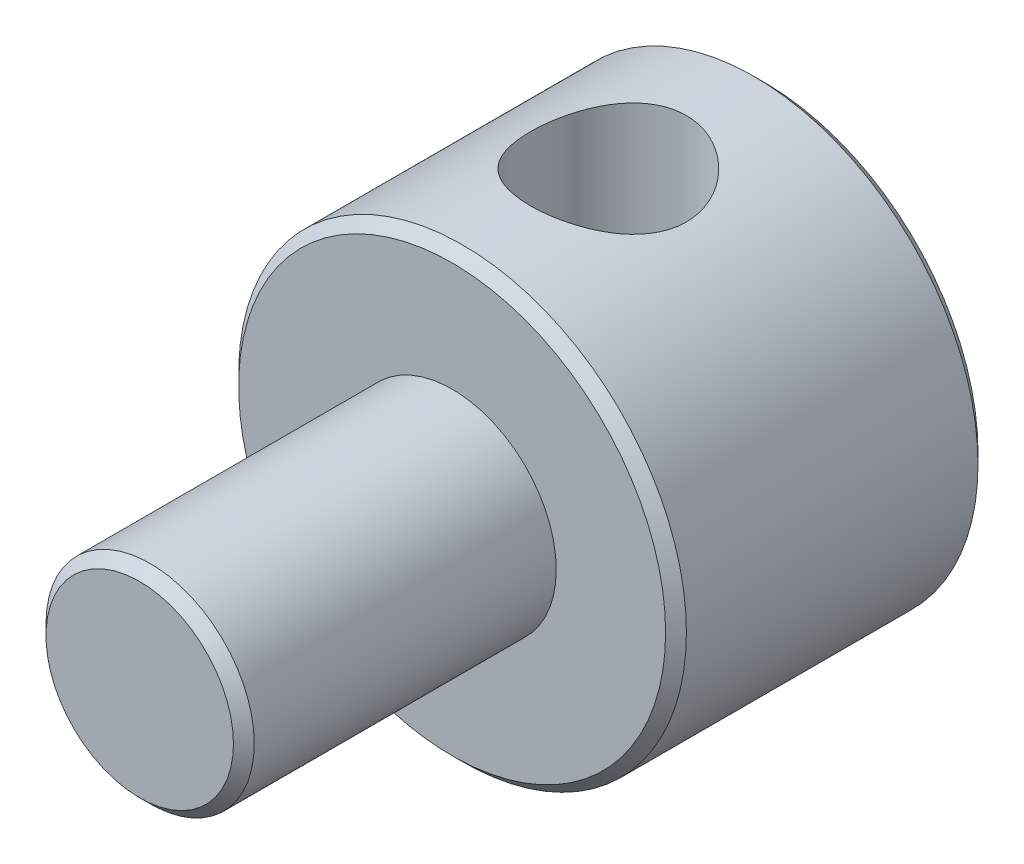
SolidWorks part; units mm, degrees
material "尼龙 101"
ref_plane "Front Plane" through (0, 0, 0) normal (0, 0, 1) x (1, 0, 0)
ref_plane "Top Plane" through (0, 0, 0) normal (0, 1, 0) x (1, 0, 0)
ref_plane "Right Plane" through (0, 0, 0) normal (1, 0, 0) x (0, 0, -1)
sketch "Sketch1" plane through (0, 0, 0) normal (0, 0, 1) x (1, 0, 0)
  circle A0 centre (0, 0) radius 4.3
  dimension "D1" = 8.6
extrude "Boss-Extrude1" add sketch "Sketch1" along normal blind 6
sketch "Sketch2" plane through (0, 0, 6) normal (0, 0, 1) x (1, 0, 0)
  circle A0 centre (0, 0) radius 2
  dimension "D1" = 4
extrude "Boss-Extrude2" add sketch "Sketch2" along normal blind 6
cosmetic thread "Cosmetic Thread1" parameters "D1"=6, "D2"=3.242
chamfer "Chamfer1" distance 0.2 angle 45 3 edges at (4.3, 0, 0) (4.3, 0, 6) (2, 0, 12)
ref_plane "Plane1" through (0, 5, 0) normal (0, 1, 0) x (1, 0, 0)
hole_wizard "Ø3.0 (3) Diameter Hole1" positions "Sketch4" profile "Sketch5" hole size "Ø3.0" standard "GB" end condition through all
sketch "Sketch4" plane through (0, 5, 0) normal (0, 1, 0) x (1, 0, 0)
  point P0 (0, -3)
  dimension "D1" = 3
sketch "Sketch5" plane through (0, 5, 3) normal (1, 0, 0) x (0, 0, 1)
  line L0 (0, 0) -> (0, 9.3)
  line L1 (0, 9.3) -> (1.5, 9.3)
  line L2 (1.5, 9.3) -> (1.5, 0)
  line L5 (1.5, 0) -> (0, 0)
  line L11 (0, -6.35) -> (0, 107.95) construction
  dimension "通孔孔直径" = 3
  dimension "通孔孔深度" = 9.3
